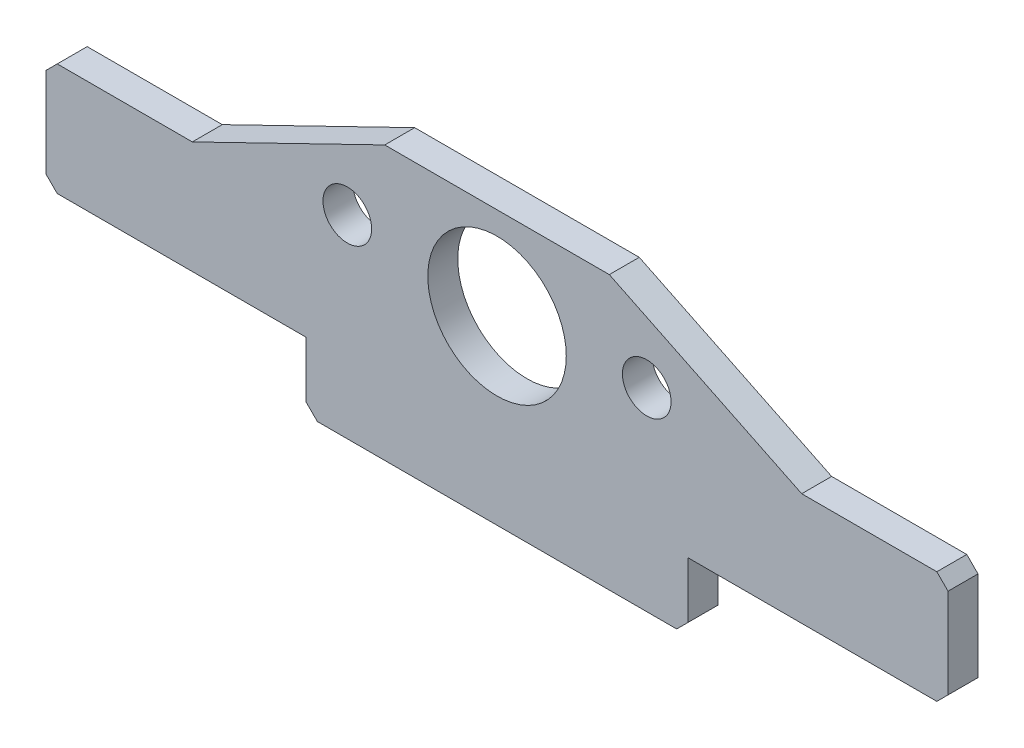
from build123d import *

# Parameters (mm, degrees)
SKETCH1_R           = 32.5
SKETCH1_R_2         = 92.5
BOSS_EXTRUDE1_DEPTH = 40


with BuildPart() as part:
    # Sketch1 → Boss-Extrude1 (new body)
    with BuildSketch(Plane.XY):
        Polygon((240, 0), (-240, 0), (-255, 15), (-255, 90), (-587.5, 90), (-602.5, 105), (-602.5, 225), (-587.5, 240), (-407, 240), (-150, 365), (150, 365), (407, 240), (587.5, 240), (602.5, 225), (602.5, 105), (587.5, 90), (255, 90), (255, 15), align=None)
        with Locations((-200, 259)):
            Circle(SKETCH1_R, mode=Mode.SUBTRACT)
        with Locations(Location((200, 259, 0), (0, 0, 180))):
            Circle(SKETCH1_R, mode=Mode.SUBTRACT)
        with Locations((0, 242)):
            Circle(SKETCH1_R_2, mode=Mode.SUBTRACT)
    extrude(amount=BOSS_EXTRUDE1_DEPTH)


solid = part.part
